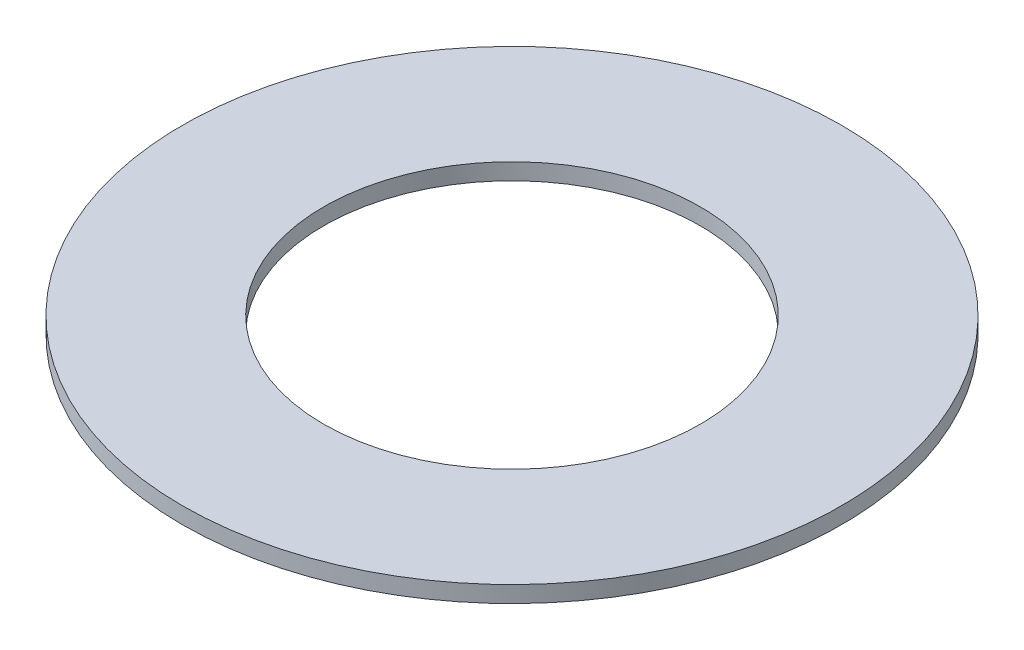
SolidWorks part; units mm, degrees
material "EPDM 60 硬度计"
ref_plane "Front Plane" through (0, 0, 0) normal (0, 0, 1) x (1, 0, 0)
ref_plane "Top Plane" through (0, 0, 0) normal (0, 1, 0) x (1, 0, 0)
ref_plane "Right Plane" through (0, 0, 0) normal (1, 0, 0) x (0, 0, -1)
sketch "Sketch1" plane through (0, 0, 0) normal (0, 1, 0) x (1, 0, 0)
  circle A0 centre (0, 0) radius 7
  circle A1 centre (0, 0) radius 4
  dimension "D1" = 14
  dimension "D2" = 8
extrude "Boss-Extrude1" add sketch "Sketch1" along normal blind 0.35
